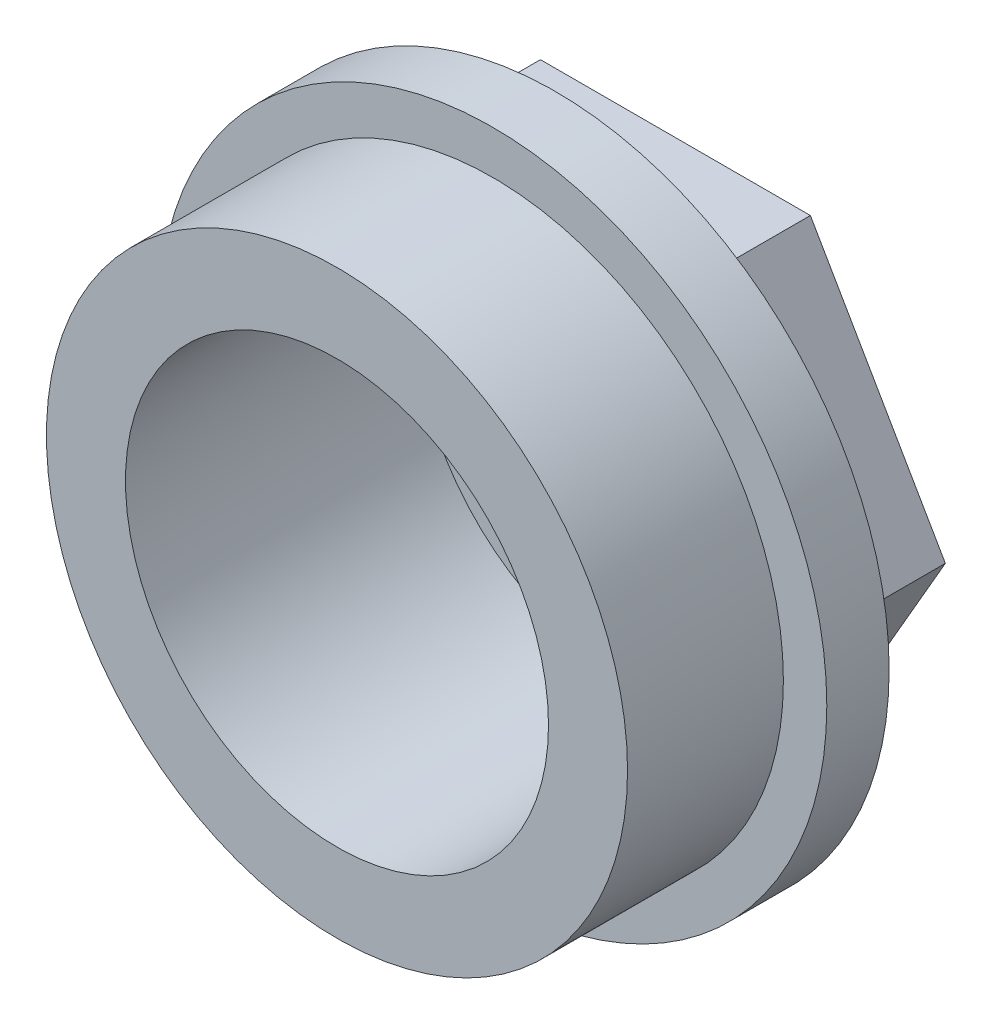
from build123d import *

# Parameters (mm, degrees)
SKETCH_1_R          = 15
EXTRUDE_1_DEPTH     = 2.8
EXTRUDE_2_DEPTH     = 5.4
SKETCH_3_R          = 13.05
EXTRUDE_3_DEPTH     = 7
SKETCH_4_R          = 9.5
CUT_EXTRUDE_1_DEPTH = 13


with BuildPart() as part:
    # 草图1 → 凸台-拉伸1 (new body)
    with BuildSketch(Plane.XY):
        Circle(SKETCH_1_R)
    extrude(amount=EXTRUDE_1_DEPTH)

    # 草图2 → 凸台-拉伸2 (add)
    with BuildSketch(Plane(origin=(0, 0, 0), x_dir=(-1, 0, 0), z_dir=(0, 0, -1))):
        Polygon((6.062177826, -10.5), (12.124355653, 0), (6.062177826, 10.5), (-6.062177826, 10.5), (-12.124355653, 0), (-6.062177826, -10.5), align=None)
    extrude(amount=EXTRUDE_2_DEPTH)

    # 草图3 → 凸台-拉伸3 (add)
    with BuildSketch(Plane.XY.offset(2.8)):
        Circle(SKETCH_3_R)
    extrude(amount=EXTRUDE_3_DEPTH)

    # 草图4 → 切除-拉伸1 (cut)
    with BuildSketch(Plane.XY.offset(9.8)):
        Circle(SKETCH_4_R)
    extrude(amount=-CUT_EXTRUDE_1_DEPTH, mode=Mode.SUBTRACT)


solid = part.part
